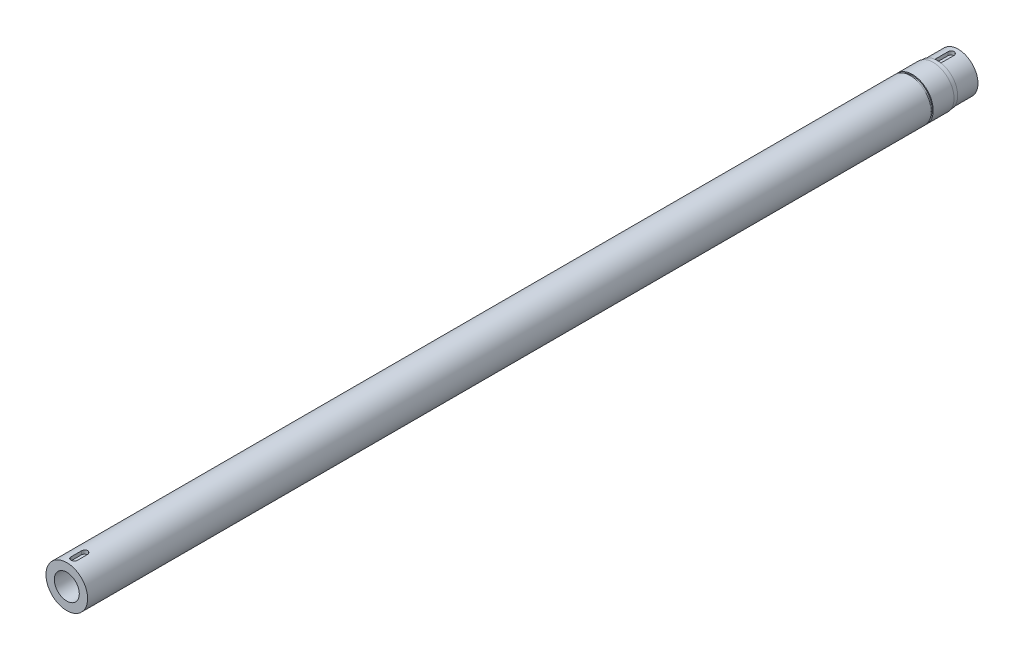
SolidWorks part; units mm, degrees
ref_plane "Front Plane" through (0, 0, 0) normal (0, 0, 1) x (1, 0, 0)
ref_plane "Top Plane" through (0, 0, 0) normal (0, 1, 0) x (1, 0, 0)
ref_plane "Right Plane" through (0, 0, 0) normal (1, 0, 0) x (0, 0, -1)
other "Configuration Table"
sketch "Sketch1" plane through (0, 0, 0) normal (0, 0, 1) x (1, 0, 0)
  circle A0 centre (0, 0) radius 6
  circle A1 centre (0, 0) radius 9.5
  dimension "D1" = 12
  dimension "D2" = 19
extrude "Boss-Extrude1" add sketch "Sketch1" along normal blind 10
ref_plane "Plane1" through (0, 9.5, 0) normal (0, 1, 0) x (1, 0, 0)
sketch "Sketch2" plane through (0, 9.5, 0) normal (0, 1, 0) x (1, 0, 0)
  line L0 (0, 0) -> (0, -12.6738) construction
  line L1 (6, 0) -> (-6, 0) construction
  line L2 (0, -3.5) -> (0, -8.5) construction
  line L3 (1.5, -3.5) -> (1.5, -8.5)
  line L4 (-1.5, -3.5) -> (-1.5, -8.5)
  line L5 (-1.5, -8.5) -> (-1.5, -10)
  line L6 (-9.5, -10) -> (9.5, -10) construction
  line L7 (-1.5, -10) -> (1.5, -10)
  line L8 (1.5, -10) -> (1.5, -8.5)
  arc A0 (1.5, -3.5) -> (-1.5, -3.5) centre (0, -3.5) ccw
  point P6 (0, -6)
  dimension "D2" = 1.5
  dimension "D1" = 5
  dimension "D3" = 3.5
extrude "Cut-Extrude1" cut sketch "Sketch2" against normal blind 1.8
ref_plane "Plane2" through (0, -9.5, 0) normal (0, 1, 0) x (1, 0, 0)
sketch "Sketch3" plane through (0, -9.5, 0) normal (0, 1, 0) x (1, 0, 0)
  line L0 (0, 0) -> (0, -10.9604) construction
  line L1 (0, -3.5) -> (0, -8.5) construction
  line L2 (1.5, -3.5) -> (1.5, -8.5)
  line L3 (-1.5, -3.5) -> (-1.5, -8.5)
  line L4 (9.5, 0) -> (-9.5, 0) construction
  line L5 (1.5, -8.5) -> (1.5, -10.0309)
  line L6 (1.5, -10.0309) -> (-1.5, -10.0309)
  line L7 (-1.5, -10.0309) -> (-1.5, -8.5)
  arc A0 (1.5, -3.5) -> (-1.5, -3.5) centre (0, -3.5) ccw
  point P5 (0, -6)
  dimension "D2" = 1.5
  dimension "D1" = 5
  dimension "D3" = 3.5
extrude "Cut-Extrude2" cut sketch "Sketch3" along normal blind 1.8
sketch "Sketch4" plane through (0, 0, 10) normal (0, 0, 1) x (1, 0, 0)
  circle A0 centre (0, 0) radius 6
  circle A1 centre (0, 0) radius 9.75
  dimension "D1" = 19.5
  dimension "D2" = 12
extrude "Boss-Extrude2" add sketch "Sketch4" along normal blind 2
sketch "Sketch5" plane through (0, 0, 12) normal (0, 0, 1) x (1, 0, 0)
  circle A0 centre (0, 0) radius 10
  dimension "D1" = 20
extrude "Boss-Extrude3" add sketch "Sketch5" along normal blind 10
sketch "Sketch6" plane through (0, 0, 22) normal (0, 0, 1) x (1, 0, 0)
  circle A0 centre (0, 0) radius 6
  dimension "D1" = 12
extrude "Cut-Extrude3" cut sketch "Sketch6" against normal through all
sketch "Sketch7" plane through (0, 0, 22) normal (0, 0, 1) x (1, 0, 0)
  circle A0 centre (0, 0) radius 6
  circle A1 centre (0, 0) radius 9.5
  dimension "D1" = 12
  dimension "D2" = 19
extrude "Boss-Extrude4" add sketch "Sketch7" along normal blind 1
sketch "Sketch8" plane through (0, 0, 23) normal (0, 0, 1) x (1, 0, 0)
  circle A0 centre (0, 0) radius 6
  circle A1 centre (0, 0) radius 10
extrude "Boss-Extrude5" add sketch "Sketch8" along normal blind 6
sketch "Sketch9" plane through (0, 0, 29) normal (0, 0, 1) x (1, 0, 0)
  circle A0 centre (0, 0) radius 6
  circle A1 centre (0, 0) radius 10
extrude "Boss-Extrude6" add sketch "Sketch9" along normal blind 150
sketch "Sketch10" plane through (0, 0, 179) normal (0, 0, 1) x (1, 0, 0)
  circle A0 centre (0, 0) radius 6
  circle A1 centre (0, 0) radius 10
extrude "Boss-Extrude7" add sketch "Sketch10" along normal blind 223
sketch "Sketch11" plane through (0, 0, 402) normal (0, 0, 1) x (1, 0, 0)
  circle A0 centre (0, 0) radius 6
  circle A1 centre (0, 0) radius 10
extrude "Boss-Extrude8" add sketch "Sketch11" along normal blind 26
ref_plane "Plane3" through (0, 10, 0) normal (0, 1, 0) x (1, 0, 0)
sketch "Sketch12" plane through (0, 10, 0) normal (0, 1, 0) x (1, 0, 0)
  line L0 (0, -419.5) -> (0, -424.5) construction
  line L1 (1.5, -419.5) -> (1.5, -424.5)
  line L2 (-1.5, -419.5) -> (-1.5, -424.5)
  line L3 (-10, -428) -> (10, -428) construction
  line L4 (-10, -428) -> (10, -428) construction
  arc A0 (1.5, -419.5) -> (-1.5, -419.5) centre (0, -419.5) ccw
  arc A1 (-1.5, -424.5) -> (1.5, -424.5) centre (0, -424.5) ccw
  point P3 (0, -422)
  dimension "D1" = 1.5
  dimension "D2" = 5
  dimension "D3" = 3.5
extrude "Cut-Extrude4" cut sketch "Sketch12" against normal blind 1.8
